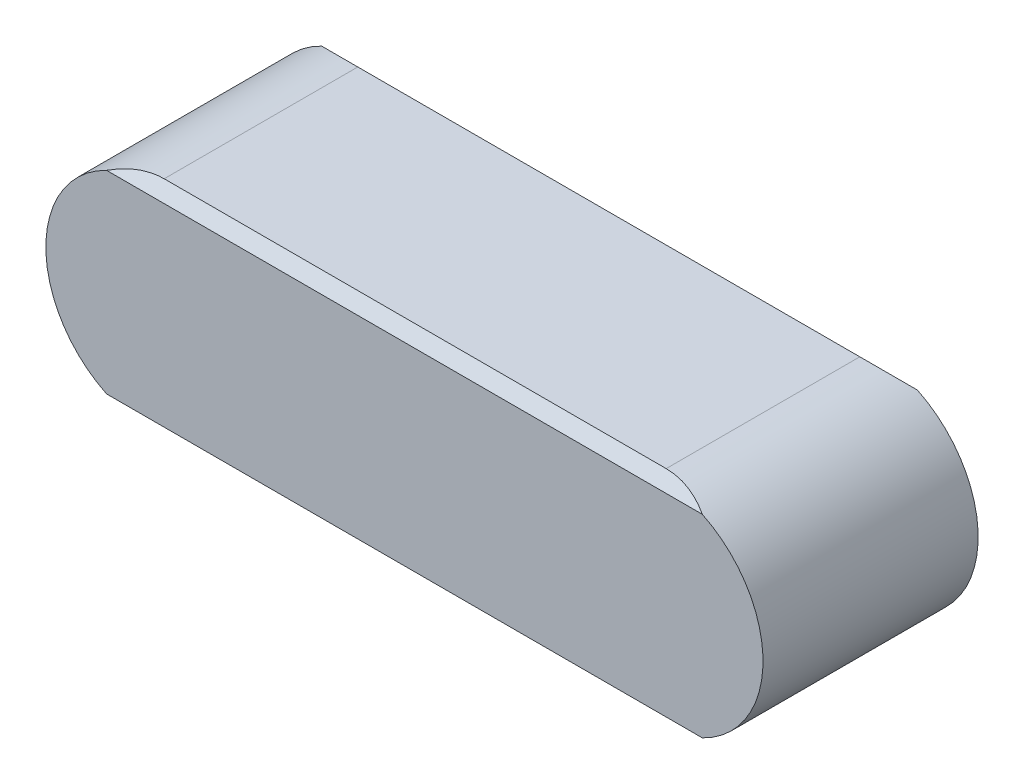
from build123d import *

# Parameters (mm, degrees)
EXTRUDE_1_DEPTH     = 6
SKETCH_2_W          = 12
SKETCH_2_H          = 12
CUT_EXTRUDE_1_DEPTH = 20


with BuildPart() as part:
    # 草图1 → 凸台-拉伸1 (new body)
    with BuildSketch(Plane.XY):
        with BuildLine():
            Line((3, 0), (17, 0))
            ThreePointArc((17, 0), (19.121320344, 0.878679656), (20, 3))
            ThreePointArc((20, 3), (19.121320344, 5.121320344), (17, 6))
            Line((17, 6), (3, 6))
            ThreePointArc((3, 6), (0.878679656, 5.121320344), (0, 3))
            ThreePointArc((0, 3), (0.878679656, 0.878679656), (3, 0))
        make_face()
    extrude(amount=EXTRUDE_1_DEPTH)

    # 草图2 → 切除-拉伸1 (cut)
    with BuildSketch(Plane(origin=(0, 0, 0), x_dir=(0, 0, -1), z_dir=(1, 0, 0))):
        with Locations((-3, 3)):
            Rectangle(SKETCH_2_W, SKETCH_2_H)
        Polygon((-6, 5.7), (-6, 0.3), (-5.7, 0), (-0.3, 0), (0, 0.3), (0, 5.7), (-0.3, 6), (-5.7, 6), align=None, mode=Mode.SUBTRACT)
    extrude(amount=CUT_EXTRUDE_1_DEPTH, mode=Mode.SUBTRACT)


solid = part.part
